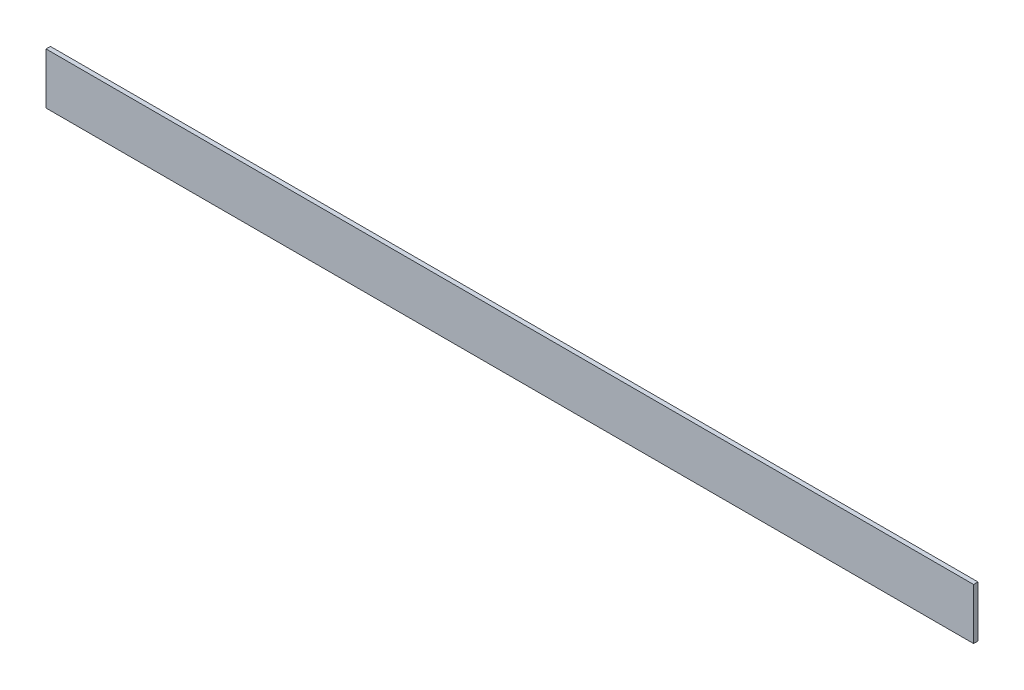
SolidWorks part; units mm, degrees
material "1023 碳钢板 (SS)"
ref_plane "前视基准面" through (0, 0, 0) normal (0, 0, 1) x (1, 0, 0)
ref_plane "上视基准面" through (0, 0, 0) normal (0, 1, 0) x (1, 0, 0)
ref_plane "右视基准面" through (0, 0, 0) normal (1, 0, 0) x (0, 0, -1)
sketch "草图1" plane through (0, 0, 0) normal (0, 0, 1) x (1, 0, 0)
  line L1 (-317, 17.5) -> (317, 17.5)
  line L2 (-317, 17.5) -> (-317, -17.5)
  line L3 (-317, -17.5) -> (317, -17.5)
  line L4 (317, 17.5) -> (317, -17.5)
  line L5 (-317, 17.5) -> (317, -17.5) construction
  line L6 (-317, -17.5) -> (317, 17.5) construction
  point P0 (0, 0)
  dimension "D1" = 634
  dimension "D2" = 35
extrude "凸台-拉伸1" add sketch "草图1" along normal blind 3
